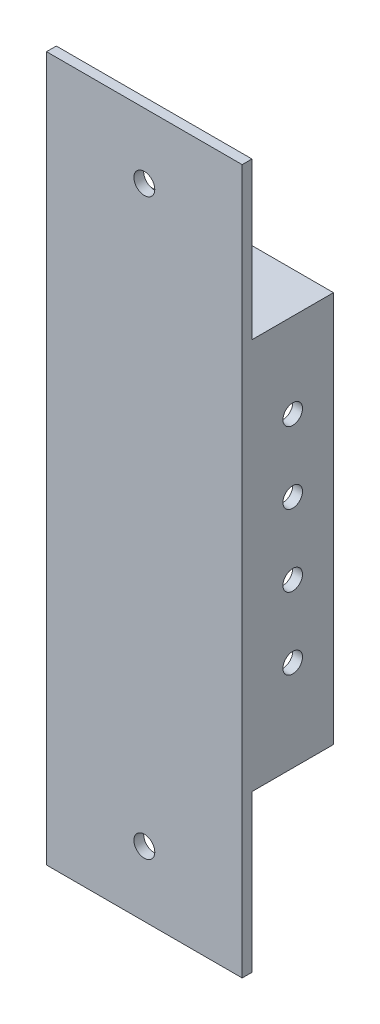
from build123d import *

# Parameters (mm, degrees)
SKETCH1_W                 = 600
SKETCH1_H                 = 1200
BOSS_EXTRUDE1_DEPTH       = 30
SKETCH3_W                 = 600
SKETCH3_H                 = 1200
SKETCH3_W_2               = 540
SKETCH3_H_2               = 1140
BOSS_EXTRUDE2_DEPTH       = 250
SKETCH4_R                 = 30
CUT_EXTRUDE2_DEPTH        = 660
LPATTERN1_COUNT           = 4
LPATTERN1_PITCH           = 220
SKETCH5_R                 = 5
CUT_EXTRUDE3_DEPTH        = 20
LPATTERN2_COUNT           = 4
LPATTERN2_PITCH           = 190
LPATTERN3_COUNT           = 4
LPATTERN3_PITCH           = 390
LPATTERN4_COPY_1_SKETCH_R = 5
LPATTERN4_COPY_1_DEPTH    = 20
LPATTERN4_COPY_2_SKETCH_R = 5
LPATTERN4_COPY_2_DEPTH    = 20
LPATTERN4_COPY_3_SKETCH_R = 5
LPATTERN4_COPY_3_DEPTH    = 20
LPATTERN4_COPY_4_SKETCH_R = 5
LPATTERN4_COPY_4_DEPTH    = 20
LPATTERN5_COPY_1_SKETCH_R = 5
LPATTERN5_COPY_1_DEPTH    = 20
LPATTERN5_COPY_2_SKETCH_R = 5
LPATTERN5_COPY_2_DEPTH    = 20
LPATTERN5_COPY_3_SKETCH_R = 5
LPATTERN5_COPY_3_DEPTH    = 20
LPATTERN5_COPY_4_SKETCH_R = 5
LPATTERN5_COPY_4_DEPTH    = 20
SKETCH6_W                 = 600
SKETCH6_H                 = 30
BOSS_EXTRUDE3_DEPTH       = 480
SKETCH8_W                 = 600
SKETCH8_H                 = 30
BOSS_EXTRUDE4_DEPTH       = 480
SKETCH9_R                 = 32
CUT_EXTRUDE4_DEPTH        = 480


with BuildPart() as part:
    # Sketch1 → Boss-Extrude1 (new body)
    with BuildSketch(Plane.XY):
        Rectangle(SKETCH1_W, SKETCH1_H)
    extrude(amount=BOSS_EXTRUDE1_DEPTH)

    # Sketch3 → Boss-Extrude2 (add)
    with BuildSketch(Plane(origin=(0, 0, 0), x_dir=(-1, 0, 0), z_dir=(0, 0, -1))):
        Rectangle(SKETCH3_W, SKETCH3_H)
        Rectangle(SKETCH3_W_2, SKETCH3_H_2, mode=Mode.SUBTRACT)
    extrude(amount=BOSS_EXTRUDE2_DEPTH)

    # Sketch4 → Cut-Extrude2 (cut)
    with BuildSketch(Plane.ZY.offset(300)):
        with Locations((-125, 340)):
            Circle(SKETCH4_R)
    cut_extrude2 = extrude(amount=-CUT_EXTRUDE2_DEPTH, mode=Mode.SUBTRACT)

    # LPattern1: Cut-Extrude2 ×4
    with Locations(*[(0, -i * LPATTERN1_PITCH, 0) for i in range(1, LPATTERN1_COUNT)]):
        add(cut_extrude2, mode=Mode.SUBTRACT)

    # Sketch5 → Cut-Extrude3 (cut)
    with BuildSketch(Plane(origin=(0, 0, -250), x_dir=(-1, 0, 0), z_dir=(0, 0, -1))):
        with Locations((-285, 585)):
            Circle(SKETCH5_R)
    cut_extrude3 = extrude(amount=-CUT_EXTRUDE3_DEPTH, mode=Mode.SUBTRACT)

    # LPattern2: Cut-Extrude3 ×4
    with Locations(*[(-i * LPATTERN2_PITCH, 0, 0) for i in range(1, LPATTERN2_COUNT)]):
        add(cut_extrude3, mode=Mode.SUBTRACT)

    # LPattern3: Cut-Extrude3 ×4
    with Locations(*[(0, -i * LPATTERN3_PITCH, 0) for i in range(1, LPATTERN3_COUNT)]):
        add(cut_extrude3, mode=Mode.SUBTRACT)

    # LPattern4 copy 1 sketch → LPattern4 copy 1 (cut)
    with BuildSketch(Plane(origin=(-570, -390, -250), x_dir=(-1, 0, 0), z_dir=(0, 0, -1))):
        with Locations((-285, 585)):
            Circle(LPATTERN4_COPY_1_SKETCH_R)
    extrude(amount=-LPATTERN4_COPY_1_DEPTH, mode=Mode.SUBTRACT)

    # LPattern4 copy 2 sketch → LPattern4 copy 2 (cut)
    with BuildSketch(Plane(origin=(-570, -780, -250), x_dir=(-1, 0, 0), z_dir=(0, 0, -1))):
        with Locations((-285, 585)):
            Circle(LPATTERN4_COPY_2_SKETCH_R)
    extrude(amount=-LPATTERN4_COPY_2_DEPTH, mode=Mode.SUBTRACT)

    # LPattern4 copy 3 sketch → LPattern4 copy 3 (cut)
    with BuildSketch(Plane(origin=(-570, -1170, -250), x_dir=(-1, 0, 0), z_dir=(0, 0, -1))):
        with Locations((-285, 585)):
            Circle(LPATTERN4_COPY_3_SKETCH_R)
    extrude(amount=-LPATTERN4_COPY_3_DEPTH, mode=Mode.SUBTRACT)

    # LPattern4 copy 4 sketch → LPattern4 copy 4 (cut)
    with BuildSketch(Plane(origin=(-570, 0, -250), x_dir=(-1, 0, 0), z_dir=(0, 0, -1))):
        with Locations((-285, 585)):
            Circle(LPATTERN4_COPY_4_SKETCH_R)
    extrude(amount=-LPATTERN4_COPY_4_DEPTH, mode=Mode.SUBTRACT)

    # LPattern5 copy 1 sketch → LPattern5 copy 1 (cut)
    with BuildSketch(Plane(origin=(-190, -1170, -250), x_dir=(-1, 0, 0), z_dir=(0, 0, -1))):
        with Locations((-285, 585)):
            Circle(LPATTERN5_COPY_1_SKETCH_R)
    extrude(amount=-LPATTERN5_COPY_1_DEPTH, mode=Mode.SUBTRACT)

    # LPattern5 copy 2 sketch → LPattern5 copy 2 (cut)
    with BuildSketch(Plane(origin=(-380, -1170, -250), x_dir=(-1, 0, 0), z_dir=(0, 0, -1))):
        with Locations((-285, 585)):
            Circle(LPATTERN5_COPY_2_SKETCH_R)
    extrude(amount=-LPATTERN5_COPY_2_DEPTH, mode=Mode.SUBTRACT)

    # LPattern5 copy 3 sketch → LPattern5 copy 3 (cut)
    with BuildSketch(Plane(origin=(-570, -1170, -250), x_dir=(-1, 0, 0), z_dir=(0, 0, -1))):
        with Locations((-285, 585)):
            Circle(LPATTERN5_COPY_3_SKETCH_R)
    extrude(amount=-LPATTERN5_COPY_3_DEPTH, mode=Mode.SUBTRACT)

    # LPattern5 copy 4 sketch → LPattern5 copy 4 (cut)
    with BuildSketch(Plane(origin=(0, -1170, -250), x_dir=(-1, 0, 0), z_dir=(0, 0, -1))):
        with Locations((-285, 585)):
            Circle(LPATTERN5_COPY_4_SKETCH_R)
    extrude(amount=-LPATTERN5_COPY_4_DEPTH, mode=Mode.SUBTRACT)

    # Sketch6 → Boss-Extrude3 (add)
    with BuildSketch(Plane.XZ.offset(600)):
        with Locations((0, 15)):
            Rectangle(SKETCH6_W, SKETCH6_H)
    extrude(amount=BOSS_EXTRUDE3_DEPTH)

    # Sketch8 → Boss-Extrude4 (add)
    with BuildSketch(Plane(origin=(0, 600, 0), x_dir=(1, 0, 0), z_dir=(0, 1, 0))):
        with Locations((0, -15)):
            Rectangle(SKETCH8_W, SKETCH8_H)
    extrude(amount=BOSS_EXTRUDE4_DEPTH)

    # Sketch9 → Cut-Extrude4 (cut)
    with BuildSketch(Plane.XY.offset(30)):
        with Locations((0, 880)):
            Circle(SKETCH9_R)
        with Locations((0, -880)):
            Circle(SKETCH9_R)
    extrude(amount=-CUT_EXTRUDE4_DEPTH, mode=Mode.SUBTRACT)


solid = part.part
